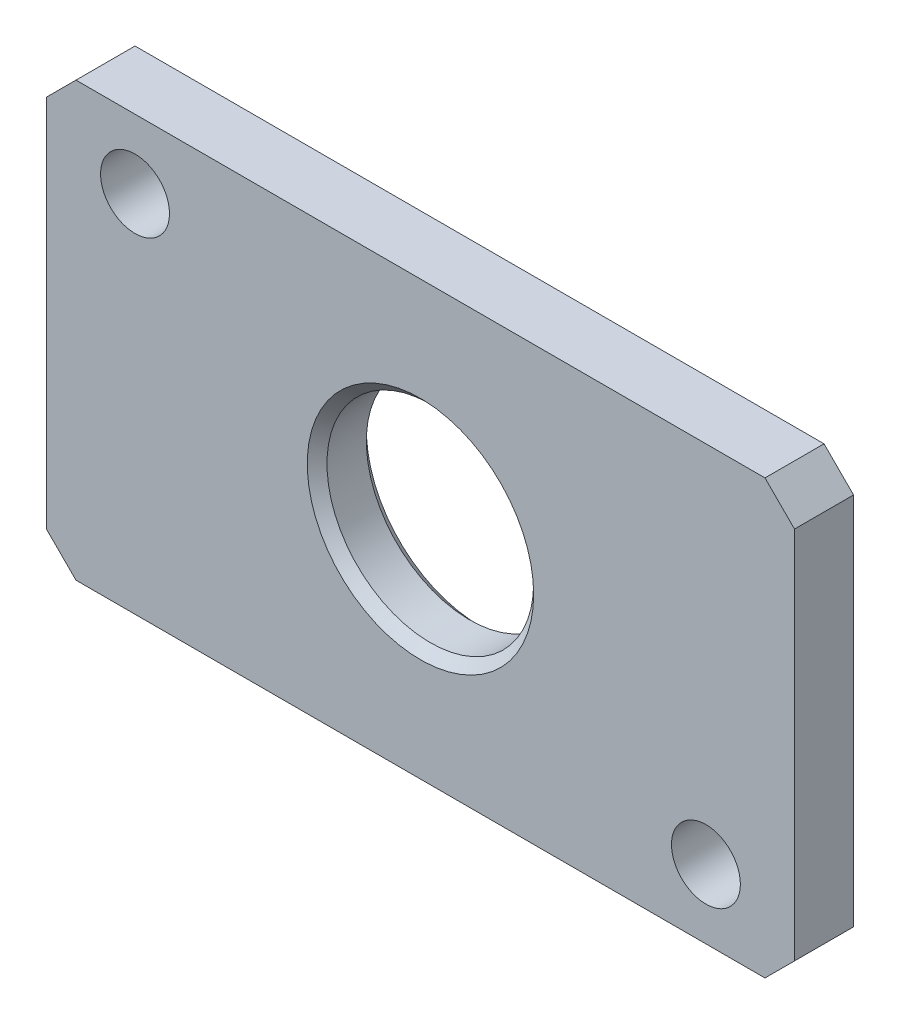
from build123d import *

# Parameters (mm, degrees)
SKETCH1_W           = 38
SKETCH1_H           = 22
SKETCH1_R           = 5.25
SKETCH1_R_2         = 1.75
BOSS_EXTRUDE1_DEPTH = 3
CHAMFER1_SIZE       = 1.5
CHAMFER2_SIZE       = 0.5


with BuildPart() as part:
    # Sketch1 → Boss-Extrude1 (new body)
    with BuildSketch(Plane.XY):
        Rectangle(SKETCH1_W, SKETCH1_H)
        Circle(SKETCH1_R, mode=Mode.SUBTRACT)
        with Locations((-14.5, 7.5)):
            Circle(SKETCH1_R_2, mode=Mode.SUBTRACT)
        with Locations((14.5, -7.5)):
            Circle(SKETCH1_R_2, mode=Mode.SUBTRACT)
    extrude(amount=BOSS_EXTRUDE1_DEPTH)

    # Chamfer1
    chamfer1_edges = [part.edges().sort_by_distance(p)[0] for p in [
        (19, -11, 1.5),
        (-19, -11, 1.5),
        (-19, 11, 1.5),
        (19, 11, 1.5),
    ]]
    chamfer(chamfer1_edges, length=CHAMFER1_SIZE)

    # Chamfer2
    chamfer2_edges = [part.edges().sort_by_distance(p)[0] for p in [
        (-5.25, 0, 0),
        (-5.25, 0, 3),
    ]]
    chamfer(chamfer2_edges, length=CHAMFER2_SIZE)


solid = part.part
